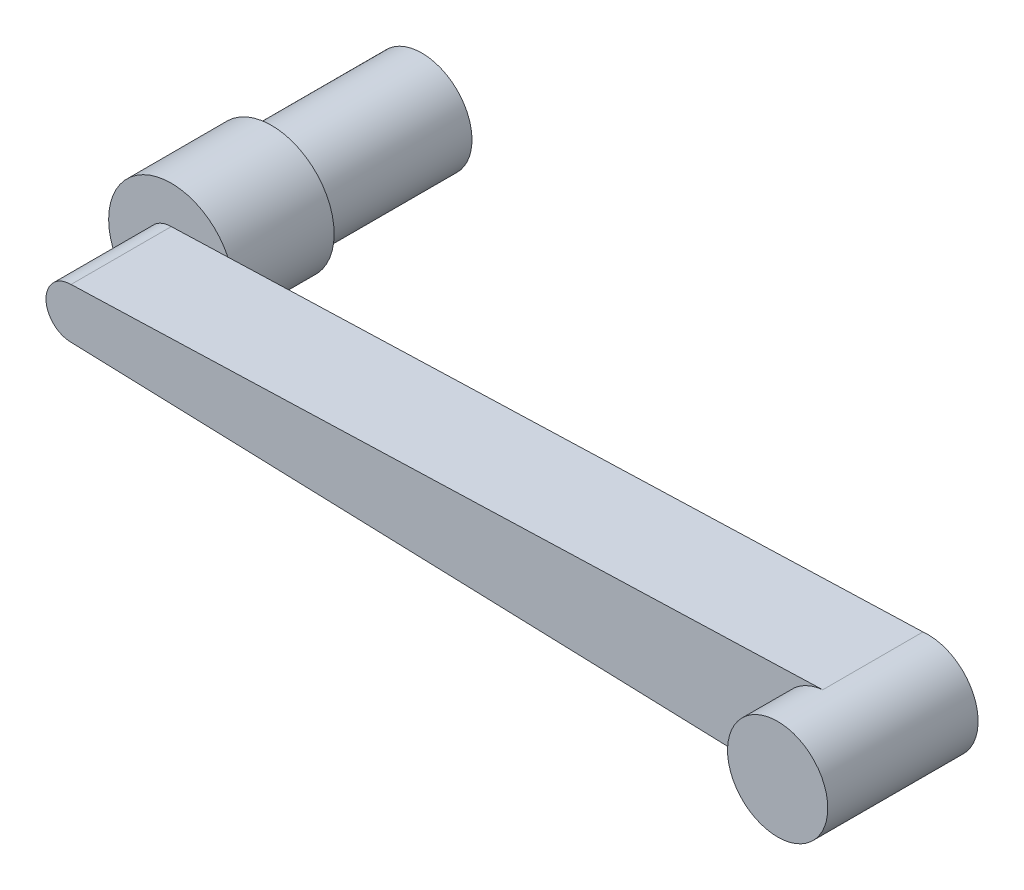
from build123d import *
from build123d.topology import SkipClean

# Parameters (mm, degrees)
SKETCH1_R           = 1.25
BOSS_EXTRUDE1_DEPTH = 1
SKETCH2_R           = 1
BOSS_EXTRUDE2_DEPTH = 1
BOSS_EXTRUDE3_DEPTH = 2
SKETCH4_R           = 1
BOSS_EXTRUDE4_DEPTH = 1
BOSS_EXTRUDE5_START = 1
SKETCH5_R           = 1.25
BOSS_EXTRUDE5_DEPTH = 1
SKETCH6_R           = 1
BOSS_EXTRUDE6_DEPTH = 3


with BuildPart() as part:
    # Sketch1 → Boss-Extrude1 (new body)
    with BuildSketch(Plane.XY):
        Circle(SKETCH1_R)
    extrude(amount=-BOSS_EXTRUDE1_DEPTH)

    # Sketch2 → Boss-Extrude2 (add)
    with BuildSketch(Plane.XY):
        Circle(SKETCH2_R)
    extrude(amount=BOSS_EXTRUDE2_DEPTH)

    # Sketch3 → Boss-Extrude3 (add)
    with BuildSketch(Plane.XY.offset(1)):
        with BuildLine():
            Line((0, 0.5), (15, 0.995012469))
            ThreePointArc((15, 0.995012469), (16.099750623, 0), (15, -0.995012469))
            Line((15, -0.995012469), (0, -0.5))
            ThreePointArc((0, -0.5), (-0.5, 0), (0, 0.5))
        make_face()
    extrude(amount=BOSS_EXTRUDE3_DEPTH)

    # Sketch4 → Boss-Extrude4 (add)
    with SkipClean():  # the faces are left unmerged after this step: merging them gives an invalid solid
        with BuildSketch(Plane.XY.offset(3)):
            with Locations(Location((15.099750623, 0, 0), (0, 0, 264.275189548))):
                Circle(SKETCH4_R)
        extrude(amount=BOSS_EXTRUDE4_DEPTH)

    # Sketch5 → Boss-Extrude5 (add)
    with SkipClean():  # the faces are left unmerged after this step: merging them gives an invalid solid
        with BuildSketch(Plane.XY.offset(BOSS_EXTRUDE5_START)):
            Circle(SKETCH5_R)
        extrude(amount=-BOSS_EXTRUDE5_DEPTH)

    # Sketch6 → Boss-Extrude6 (add)
    with SkipClean():  # the faces are left unmerged after this step: merging them gives an invalid solid
        with BuildSketch(Plane(origin=(0, 0, -1), x_dir=(-1, 0, 0), z_dir=(0, 0, -1))):
            Circle(SKETCH6_R)
        extrude(amount=BOSS_EXTRUDE6_DEPTH)


solid = part.part
